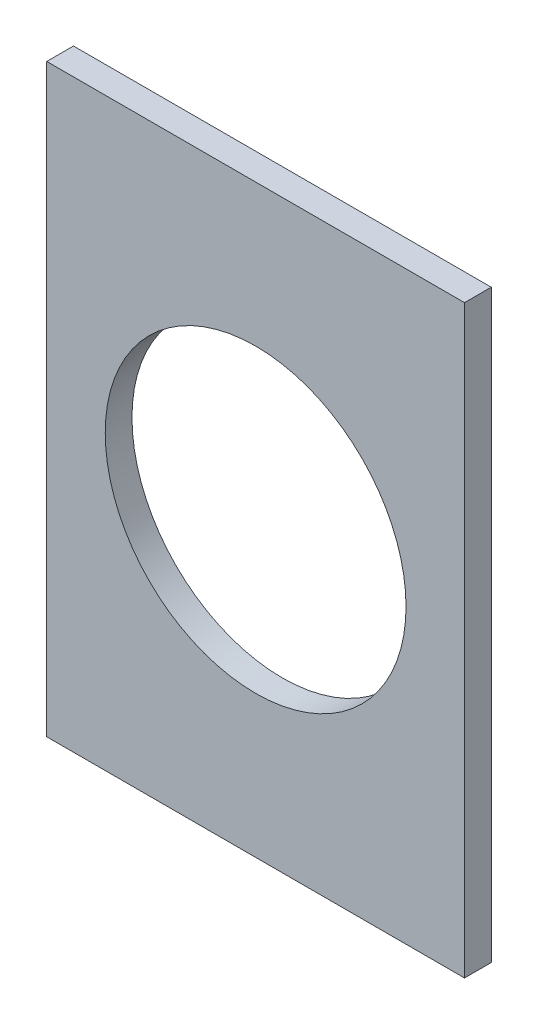
from build123d import *

# Parameters (mm, degrees)
SKETCH_1_W      = 250
SKETCH_1_H      = 350
SKETCH_1_R      = 90
EXTRUDE_1_DEPTH = 16


with BuildPart() as part:
    # 草图1 → 凸台-拉伸1 (new body)
    with BuildSketch(Plane.XY):
        Rectangle(SKETCH_1_W, SKETCH_1_H)
        Circle(SKETCH_1_R, mode=Mode.SUBTRACT)
    extrude(amount=EXTRUDE_1_DEPTH)


solid = part.part
